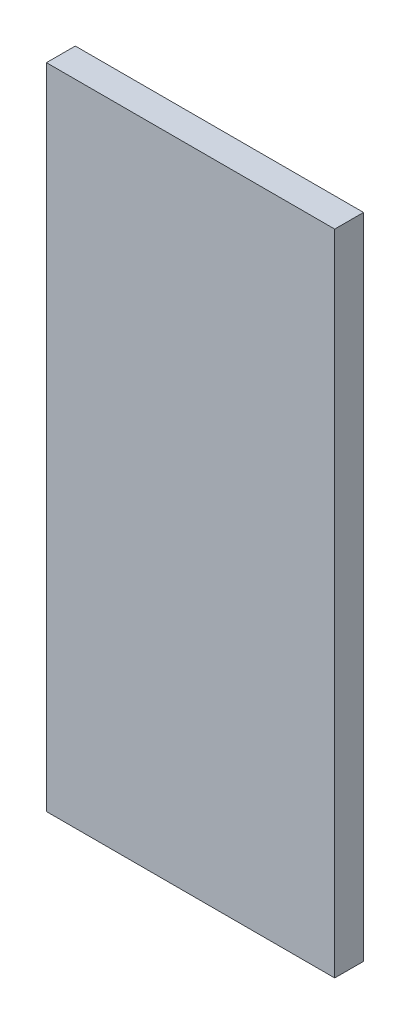
from build123d import *

# Parameters (mm, degrees)
SKETCH_1_W      = 80
SKETCH_1_H      = 180
EXTRUDE_1_DEPTH = 8


with BuildPart() as part:
    # 草图1 → 凸台-拉伸1 (new body)
    with BuildSketch(Plane.XY):
        with Locations((40, 90)):
            Rectangle(SKETCH_1_W, SKETCH_1_H)
    extrude(amount=-EXTRUDE_1_DEPTH)


solid = part.part
